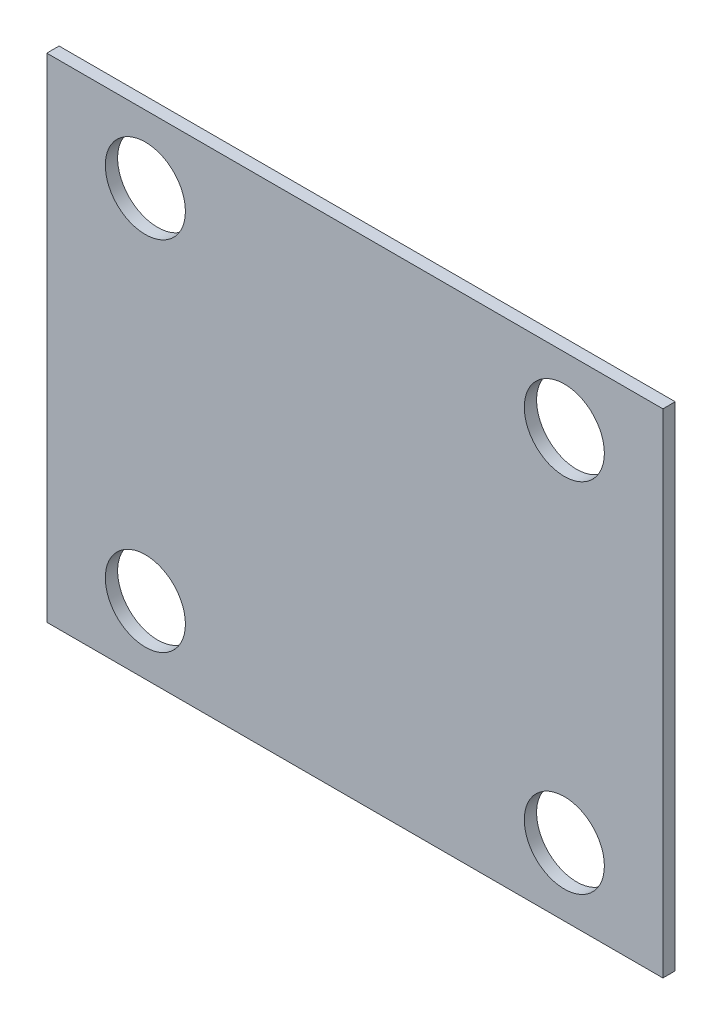
from build123d import *

# Parameters (mm, degrees)
SKETCH_1_W          = 100
SKETCH_1_H          = 80
EXTRUDE_1_DEPTH     = 2
SKETCH_2_R          = 6.5
CUT_EXTRUDE_1_DEPTH = 2


with BuildPart() as part:
    # 草图1 → 凸台-拉伸1 (new body)
    with BuildSketch(Plane.XY):
        Rectangle(SKETCH_1_W, SKETCH_1_H)
    extrude(amount=EXTRUDE_1_DEPTH)

    # 草图2 → 切除-拉伸1 (cut)
    with BuildSketch(Plane.XY.offset(2)):
        with Locations((-34, 29)):
            Circle(SKETCH_2_R)
        with Locations((34, 29)):
            Circle(SKETCH_2_R)
        with Locations((34, -29)):
            Circle(SKETCH_2_R)
        with Locations((-34, -29)):
            Circle(SKETCH_2_R)
    extrude(amount=-CUT_EXTRUDE_1_DEPTH, mode=Mode.SUBTRACT)


solid = part.part
